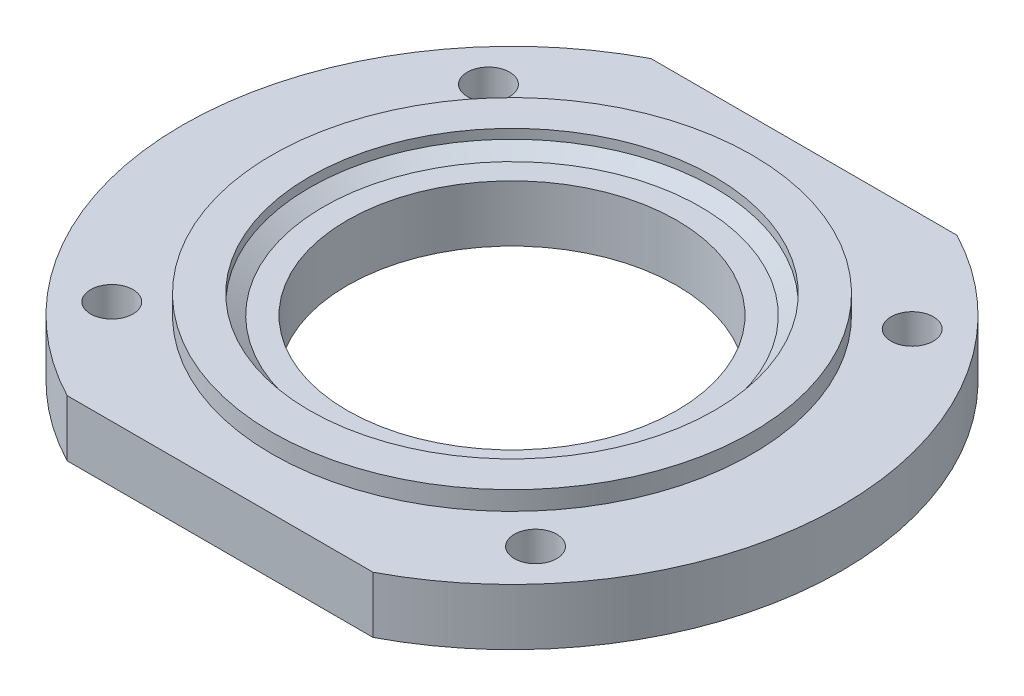
SolidWorks part; units mm, degrees
material "A6061"
ref_plane "Front Plane" through (0, 0, 0) normal (0, 0, 1) x (1, 0, 0)
ref_plane "Top Plane" through (0, 0, 0) normal (0, 1, 0) x (1, 0, 0)
ref_plane "Right Plane" through (0, 0, 0) normal (1, 0, 0) x (0, 0, -1)
sketch "Sketch1" plane through (0, 0, 0) normal (0, 0, 1) x (1, 0, 0)
  line L0 (0, 112.4312) -> (0, 12.6839) construction
  line L1 (17.5, 0) -> (35, 0)
  line L2 (35, 0) -> (35, 6)
  line L3 (25.5, 8) -> (21.5, 8)
  line L4 (21.5, 8) -> (21.5, 7)
  line L5 (21.5, 7) -> (20, 6)
  line L6 (20, 6) -> (17.5, 6)
  line L7 (0, 9.617) -> (0, -102.0412) construction
  line L8 (25.5, 8) -> (25.5, 6)
  line L9 (25.5, 6) -> (35, 6)
  line L10 (17.5, 0) -> (17.5, 6)
  dimension "D1" = 6
  dimension "D7" = 1.5
  dimension "D2" = 17.5
  dimension "D3" = 17.5
  dimension "D4" = 8
  dimension "D5" = 4
  dimension "D6" = 1
  dimension "D8" = 25.5
revolve "Revolve1" add sketch "Sketch1" angle 360 about L0
hole_wizard "Ø4.5 (4.5) Diameter Hole1" positions "Sketch3" profile "Sketch2" hole size "Ø4.5" standard "Gb"
sketch "Sketch3" plane through (0, 0, 0) normal (0, -1, 0) x (-1, 0, 0)
  line L0 (-45.8266, 0) -> (49.3445, 0) construction
  line L3 (0, 38.7545) -> (0, -40.4359) construction
  point P28 (-22.5, 20)
  point P30 (-22.5, -20)
  point P32 (22.5, 20)
  point P34 (22.5, -20)
  dimension "D1" = 40
  dimension "D2" = 45
sketch "Sketch2" plane through (22.5, 0, -20) normal (1, 0, 0) x (0, 0, -1)
  line L0 (0, 0) -> (0, 19.3519)
  line L1 (0, 19.3519) -> (2.25, 18)
  line L2 (2.25, 18) -> (2.25, 0)
  line L5 (2.25, 0) -> (0, 0)
  line L10 (0, 19.3519) -> (-2.25, 18) construction
  line L11 (0, -6.35) -> (0, 107.95) construction
  dimension "孔直径" = 4.5
  dimension "孔深度" = 18
  dimension "导头角度" = 118
sketch "Sketch4" plane through (0, 0, 0) normal (0, -1, 0) x (1, 0, 0)
  line L1 (41.7824, -31) -> (-41.7824, -31)
  line L2 (41.7824, -31) -> (41.7824, 31)
  line L3 (41.7824, 31) -> (-41.7824, 31)
  line L4 (-41.7824, -31) -> (-41.7824, 31)
  line L5 (41.7824, -31) -> (-41.7824, 31) construction
  line L6 (41.7824, 31) -> (-41.7824, -31) construction
  point P0 (0, 0)
  dimension "D1" = 62
extrude "Cut-Extrude1" cut sketch "Sketch4" against normal through all flip side to cut
